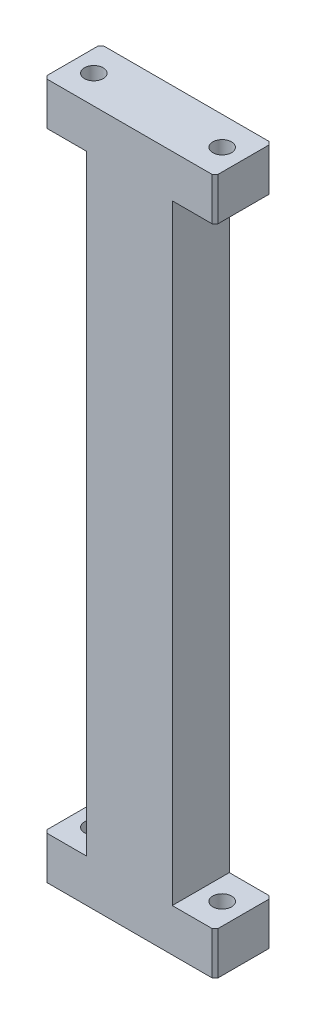
from build123d import *

# Parameters (mm, degrees)
SKETCH1_W            = 60
SKETCH1_H            = 244
BOSS_EXTRUDE1_DEPTH  = 20
SKETCH2_W            = 15
SKETCH2_H            = 214
CUT_EXTRUDE1_DEPTH   = 128.21635115
M6_CLEARANCE_HOLE1_D = 6.6
CHAMFER1_SIZE        = 1


with BuildPart() as part:
    # Sketch1 → Boss-Extrude1 (new body)
    with BuildSketch(Plane.XY):
        Rectangle(SKETCH1_W, SKETCH1_H)
    extrude(amount=BOSS_EXTRUDE1_DEPTH)

    # Sketch2 → Cut-Extrude1 (cut, through all)
    with BuildSketch(Plane.XY.offset(20)):
        with Locations((-22.5, 0)):
            Rectangle(SKETCH2_W, SKETCH2_H)
        with Locations((22.5, 0)):
            Rectangle(SKETCH2_W, SKETCH2_H)
    extrude(amount=-CUT_EXTRUDE1_DEPTH, mode=Mode.SUBTRACT)

    # M6 Clearance Hole1 (through all)
    with Locations(Plane(origin=(0, 122, 0), x_dir=(1, 0, 0), z_dir=(0, 1, 0))):
        with Locations((-22.5, -10), (22.5, -10)):
            Hole(M6_CLEARANCE_HOLE1_D / 2)

    # Chamfer1
    chamfer1_edges = [part.edges().sort_by_distance(p)[0] for p in [
        (-30, 114.5, 20),
        (30, 114.5, 0),
        (-30, -114.5, 0),
        (30, 114.5, 20),
        (-30, -114.5, 20),
        (30, -114.5, 20),
        (-30, 114.5, 0),
        (30, -114.5, 0),
    ]]
    chamfer(chamfer1_edges, length=CHAMFER1_SIZE)


solid = part.part
